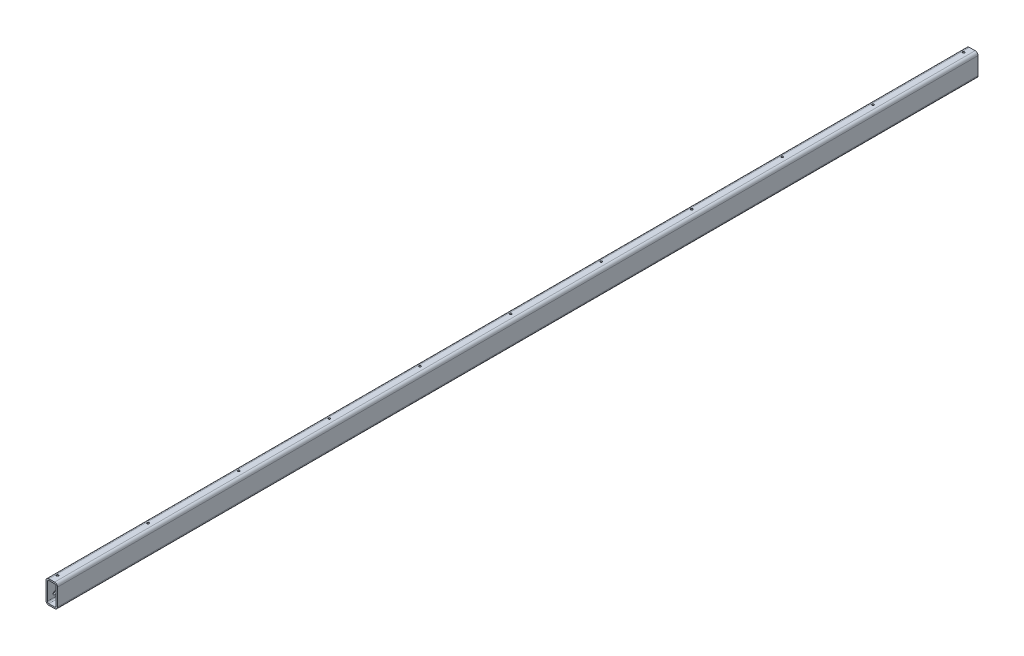
SolidWorks part; units mm, degrees
material "Q235B"
ref_plane "Plane1" through (0, 0, 0) normal (0, 0, 1) x (1, 0, 0)
ref_plane "Plane2" through (0, 0, 0) normal (0, 1, 0) x (1, 0, 0)
ref_plane "Plane3" through (0, 0, 0) normal (1, 0, 0) x (0, 0, -1)
sketch "Sketch1" plane through (0, 0, 0) normal (0, 0, 1) x (1, 0, 0)
  line L0 (-10, -35) -> (10, -35)
  line L1 (-15, -30) -> (-15, 30)
  line L2 (10, 35) -> (-10, 35)
  line L3 (15, 30) -> (15, -30)
  line L4 (-10, -40) -> (10, -40)
  line L5 (-20, -30) -> (-20, 30)
  line L6 (10, 40) -> (-10, 40)
  line L7 (20, 30) -> (20, -30)
  arc A0 (20, 30) -> (10, 40) centre (10, 30) ccw
  arc A1 (10, -40) -> (20, -30) centre (10, -30) ccw
  arc A2 (-20, -30) -> (-10, -40) centre (-10, -30) ccw
  arc A3 (-10, 40) -> (-20, 30) centre (-10, 30) ccw
  arc A4 (-10, 35) -> (-15, 30) centre (-10, 30) ccw
  arc A5 (15, 30) -> (10, 35) centre (10, 30) ccw
  arc A6 (10, -35) -> (15, -30) centre (10, -30) ccw
  arc A7 (-15, -30) -> (-10, -35) centre (-10, -30) ccw
  point P0 (0, 40)
  point P1 (20, 0)
  point P2 (0, -40)
  point P3 (-20, 0)
  point P4 (-20, 40)
  point P5 (20, 40)
  point P6 (20, -40)
  point P7 (-20, -40)
  point P8 (0, 0)
extrude "Boss-Extrude1" add sketch "Sketch1" along normal blind 3200 contours L5 A3 L6 A0 L7 A1 L4 A2 | L1 A4 L2 A5 L3 A6 L0 A7
sketch "草图1" plane through (0, 40, 0) normal (0, 1, 0) x (1, 0, 0)
  line L0 (10, -3200) -> (-10, -3200) construction
  line L1 (-20, -3200) -> (-20, 0) construction
  circle A0 centre (-5, -3175) radius 3.25
  circle A1 centre (-5, -2860) radius 3.25
  circle A2 centre (-5, -2545) radius 3.25
  circle A3 centre (-5, -2230) radius 3.25
  circle A4 centre (-5, -1915) radius 3.25
  circle A5 centre (-5, -1600) radius 3.25
  circle A6 centre (-5, -1285) radius 3.25
  circle A7 centre (-5, -970) radius 3.25
  circle A8 centre (-5, -655) radius 3.25
  circle A9 centre (-5, -340) radius 3.25
  circle A10 centre (-5, -25) radius 3.25
  dimension "D1" = 6.5
  dimension "D2" = 25
  dimension "D3" = 15
  dimension "D5" = 315
  dimension "D4" = 11
extrude "Cut-Extrude1" cut sketch "草图1" against normal blind 10
hole_wizard "M8 Tapped Hole1" positions "Sketch4" profile "Sketch5" tap size "M8" standard "GB"
sketch "Sketch4" plane through (0, 40, 0) normal (0, 1, 0) x (1, 0, 0)
  point P8 (-5, -3175)
  point P11 (-5, -2860)
  point P14 (-5, -2545)
  point P17 (-5, -2230)
  point P20 (-5, -1915)
  point P23 (-5, -1600)
  point P26 (-5, -1285)
  point P29 (-5, -970)
  point P32 (-5, -655)
  point P35 (-5, -340)
  point P38 (-5, -25)
sketch "Sketch5" plane through (-5, 40, 3175) normal (1, 0, 0) x (0, 0, 1)
  line L0 (0, 0) -> (0, 24.2929)
  line L1 (0, 24.2929) -> (3.4, 22.25)
  line L2 (3.4, 22.25) -> (3.4, 0)
  line L5 (3.4, 0) -> (0, 0)
  line L10 (0, 24.2929) -> (-3.4, 22.25) construction
  line L11 (0, -6.35) -> (0, 107.95) construction
  dimension "螺纹孔钻头直径" = 6.8
  dimension "螺纹孔钻头深度" = 22.25
  dimension "导头角度" = 118
cosmetic thread "Cosmetic Thread14" parameters "D1"=5, "D2"=8
cosmetic thread "Cosmetic Thread15" parameters "D1"=5, "D2"=8
cosmetic thread "Cosmetic Thread16" parameters "D1"=5, "D2"=8
cosmetic thread "Cosmetic Thread17" parameters "D1"=5, "D2"=8
cosmetic thread "Cosmetic Thread18" parameters "D1"=5, "D2"=8
cosmetic thread "Cosmetic Thread19" parameters "D1"=5, "D2"=8
cosmetic thread "Cosmetic Thread20" parameters "D1"=5, "D2"=8
cosmetic thread "Cosmetic Thread21" parameters "D1"=5, "D2"=8
cosmetic thread "Cosmetic Thread22" parameters "D1"=5, "D2"=8
cosmetic thread "Cosmetic Thread23" parameters "D1"=5, "D2"=8
cosmetic thread "Cosmetic Thread24" parameters "D1"=5, "D2"=8
sketch "Sketch9" plane through (-20, 0, 0) normal (-1, 0, 0) x (0, 0, 1)
  line L0 (0, -30) -> (0, 30) construction
  line L1 (3200, -40) -> (0, -40) construction
  circle A0 centre (25, -17.5) radius 5.5
  dimension "D1" = 11
  dimension "D2" = 25
  dimension "D3" = 22.5
extrude "Cut-Extrude2" cut sketch "Sketch9" against normal blind 10
pattern_linear "LPattern1" count 11 spacing 315 along (0, 0, 1) of "Cut-Extrude2"
